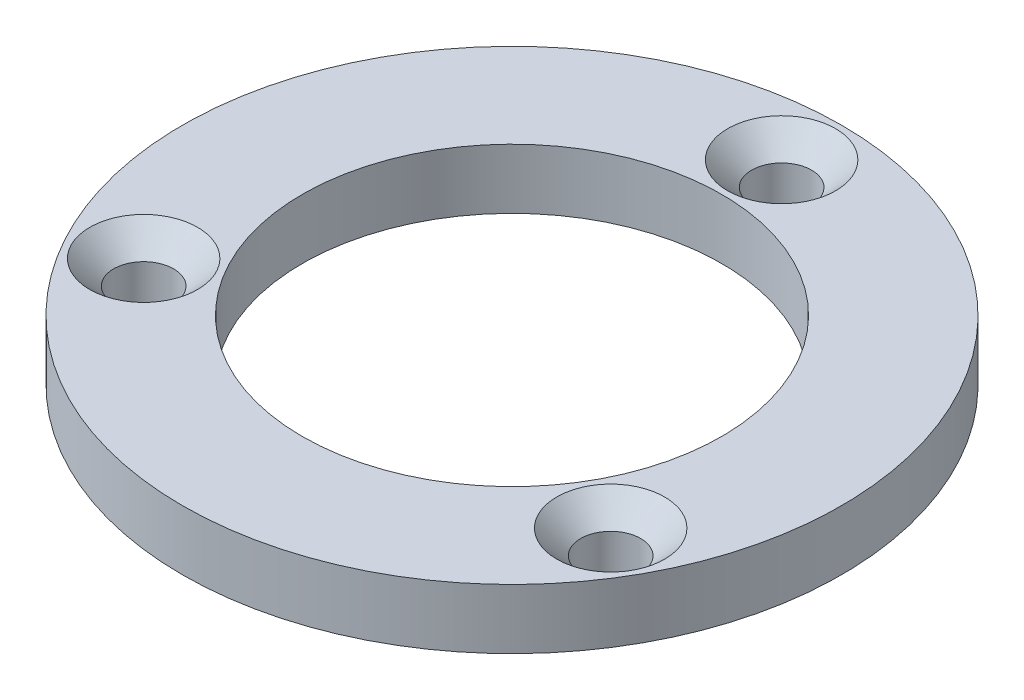
from build123d import *

# Parameters (mm, degrees)
SKETCH1_R           = 27.5
SKETCH1_R_2         = 17.5
BOSS_EXTRUDE1_DEPTH = 5
HOLE1_D             = 5
HOLE1_CSINK_D       = 9
HOLE1_CSINK_ANGLE   = 90


with BuildPart() as part:
    # Sketch1 → Boss-Extrude1 (new body)
    with BuildSketch(Plane(origin=(0, 0, 0), x_dir=(1, 0, 0), z_dir=(0, 1, 0))):
        with Locations(Location((0, 0, 0), (0, 0, 270))):
            Circle(SKETCH1_R)
        with Locations(Location((0, 0, 0), (0, 0, 270))):
            Circle(SKETCH1_R_2, mode=Mode.SUBTRACT)
    extrude(amount=BOSS_EXTRUDE1_DEPTH)

    # Hole1 (through all)
    with Locations(Plane(origin=(0, 5, 0), x_dir=(1, 0, 0), z_dir=(0, 1, 0))):
        with Locations((-19.485571585, -11.25), (0, 22.5), (19.485571585, -11.25)):
            CounterSinkHole(HOLE1_D / 2, HOLE1_CSINK_D / 2, counter_sink_angle=HOLE1_CSINK_ANGLE)


solid = part.part
